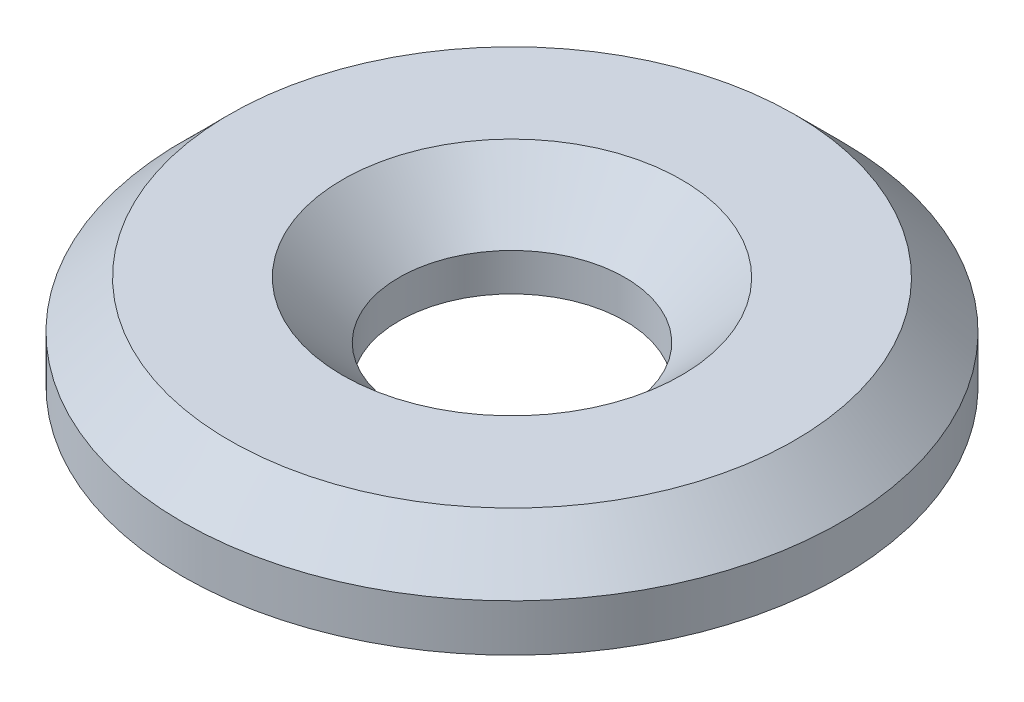
from build123d import *

# Parameters (mm, degrees)
CHAMFER1_SIZE = 2.5


with BuildPart() as part:
    # Sketch1 → Revolve1 (revolve)
    with BuildSketch(Plane.XY, mode=Mode.PRIVATE) as revolve1_sk:
        Polygon((9, 7.038461538), (17.5, 7.038461538), (17.5, 2.038461538), (6, 2.038461538), (6, 4.038461538), align=None)
    revolve(revolve1_sk.sketch.rotate(Axis((0, 7.038461538, 0), (0, -1, 0)), 90), axis=Axis((0, 7.038461538, 0), (0, -1, 0)))

    # Chamfer1
    chamfer1_edges = [part.edges().sort_by_distance(p)[0] for p in [
        (0, 7.038461538, -17.5),
    ]]
    chamfer(chamfer1_edges, length=CHAMFER1_SIZE)


solid = part.part
